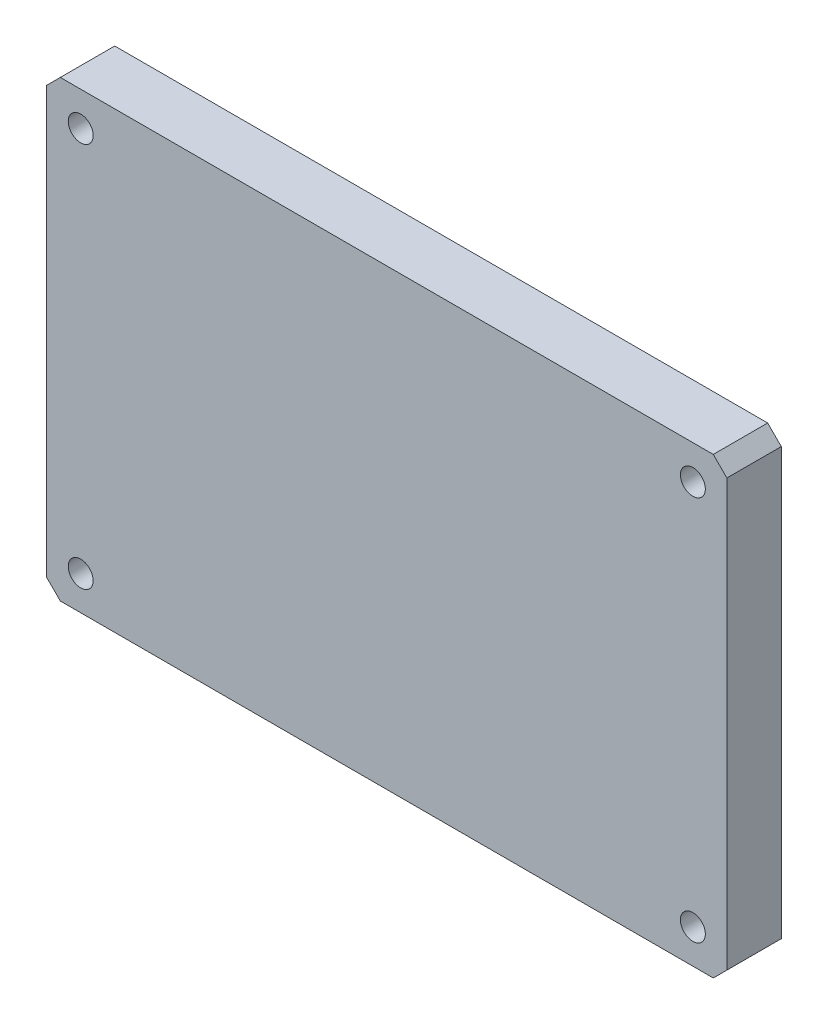
from build123d import *

# Parameters (mm, degrees)
SKETCH1_W                                         = 150
SKETCH1_H                                         = 100
BOSS_EXTRUDE1_DEPTH                               = 12
CUT_EXTRUDE3_DEPTH                                = 1
CHAMFER1_SIZE                                     = 3
HOLE_SIZE_BASED_SOCKET_HEAD_CAP_SCREW_D           = 5.5
HOLE_SIZE_BASED_SOCKET_HEAD_CAP_SCREW_CBORE_D     = 10
HOLE_SIZE_BASED_SOCKET_HEAD_CAP_SCREW_CBORE_DEPTH = 5.7


with BuildPart() as part:
    # Sketch1 → Boss-Extrude1 (new body)
    with BuildSketch(Plane.XY):
        Rectangle(SKETCH1_W, SKETCH1_H)
    extrude(amount=BOSS_EXTRUDE1_DEPTH)

    # Sketch5 → Cut-Extrude3 (cut)
    with BuildSketch(Plane(origin=(0, 0, 0), x_dir=(-1, 0, 0), z_dir=(0, 0, -1))):
        with BuildLine():
            Line((-56.0087044, -40.651312408), (-56.0087044, -24.051312408))
            ThreePointArc((-56.0087044, -24.051312408), (-56.067283044, -23.909891052), (-56.2087044, -23.851312408))
            Line((-56.2087044, -23.851312408), (-64.8087044, -23.851312408))
            ThreePointArc((-64.8087044, -23.851312408), (-64.950125756, -23.792733764), (-65.0087044, -23.651312408))
            Line((-65.0087044, -23.651312408), (-65.0087044, -17.651312408))
            ThreePointArc((-65.0087044, -17.651312408), (-64.950125756, -17.509891052), (-64.8087044, -17.451312408))
            Line((-64.8087044, -17.451312408), (-60.6087044, -17.451312408))
            ThreePointArc((-60.6087044, -17.451312408), (-60.467283044, -17.392733764), (-60.4087044, -17.251312408))
            Line((-60.4087044, -17.251312408), (-60.4087044, 4.948687592))
            ThreePointArc((-60.4087044, 4.948687592), (-60.467283044, 5.090108948), (-60.6087044, 5.148687592))
            Line((-60.6087044, 5.148687592), (-64.8087044, 5.148687592))
            ThreePointArc((-64.8087044, 5.148687592), (-64.950125756, 5.207266236), (-65.0087044, 5.348687592))
            Line((-65.0087044, 5.348687592), (-65.0087044, 11.348687592))
            ThreePointArc((-65.0087044, 11.348687592), (-64.950125756, 11.490108948), (-64.8087044, 11.548687592))
            Line((-64.8087044, 11.548687592), (-59.2087044, 11.548687592))
            ThreePointArc((-59.2087044, 11.548687592), (-59.067283044, 11.607266236), (-59.0087044, 11.748687592))
            Line((-59.0087044, 11.748687592), (-59.0087044, 36.248687592))
            ThreePointArc((-59.0087044, 36.248687592), (-58.950125756, 36.390108948), (-58.8087044, 36.448687592))
            Line((-58.8087044, 36.448687592), (-43.7087044, 36.448687592))
            ThreePointArc((-43.7087044, 36.448687592), (-43.567283044, 36.507266236), (-43.5087044, 36.648687592))
            Line((-43.5087044, 36.648687592), (-43.5087044, 39.648687592))
            ThreePointArc((-43.5087044, 39.648687592), (-43.450125756, 39.790108948), (-43.3087044, 39.848687592))
            Line((-43.3087044, 39.848687592), (-37.3087044, 39.848687592))
            ThreePointArc((-37.3087044, 39.848687592), (-37.167283044, 39.790108948), (-37.1087044, 39.648687592))
            Line((-37.1087044, 39.648687592), (-37.1087044, 36.648687592))
            ThreePointArc((-37.1087044, 36.648687592), (-37.050125756, 36.507266236), (-36.9087044, 36.448687592))
            Line((-36.9087044, 36.448687592), (-4.7087044, 36.448687592))
            ThreePointArc((-4.7087044, 36.448687592), (-4.567283044, 36.507266236), (-4.5087044, 36.648687592))
            Line((-4.5087044, 36.648687592), (-4.5087044, 39.648687592))
            ThreePointArc((-4.5087044, 39.648687592), (-4.450125756, 39.790108948), (-4.3087044, 39.848687592))
            Line((-4.3087044, 39.848687592), (1.6912956, 39.848687592))
            ThreePointArc((1.6912956, 39.848687592), (1.832716956, 39.790108948), (1.8912956, 39.648687592))
            Line((1.8912956, 39.648687592), (1.8912956, 36.648687592))
            ThreePointArc((1.8912956, 36.648687592), (1.949874244, 36.507266236), (2.0912956, 36.448687592))
            Line((2.0912956, 36.448687592), (40.2912956, 36.448687592))
            ThreePointArc((40.2912956, 36.448687592), (40.432716956, 36.507266236), (40.4912956, 36.648687592))
            Line((40.4912956, 36.648687592), (40.4912956, 39.648687592))
            ThreePointArc((40.4912956, 39.648687592), (40.549874244, 39.790108948), (40.6912956, 39.848687592))
            Line((40.6912956, 39.848687592), (46.6912956, 39.848687592))
            ThreePointArc((46.6912956, 39.848687592), (46.832716956, 39.790108948), (46.8912956, 39.648687592))
            Line((46.8912956, 39.648687592), (46.8912956, 36.648687592))
            ThreePointArc((46.8912956, 36.648687592), (46.949874244, 36.507266236), (47.0912956, 36.448687592))
            Line((47.0912956, 36.448687592), (62.1912956, 36.448687592))
            ThreePointArc((62.1912956, 36.448687592), (62.332716956, 36.390108948), (62.3912956, 36.248687592))
            Line((62.3912956, 36.248687592), (62.3912956, 11.748687592))
            ThreePointArc((62.3912956, 11.748687592), (62.449874244, 11.607266236), (62.5912956, 11.548687592))
            Line((62.5912956, 11.548687592), (68.1912956, 11.548687592))
            ThreePointArc((68.1912956, 11.548687592), (68.332716956, 11.490108948), (68.3912956, 11.348687592))
            Line((68.3912956, 11.348687592), (68.3912956, 5.348687592))
            ThreePointArc((68.3912956, 5.348687592), (68.332716956, 5.207266236), (68.1912956, 5.148687592))
            Line((68.1912956, 5.148687592), (62.5912956, 5.148687592))
            ThreePointArc((62.5912956, 5.148687592), (62.449874244, 5.090108948), (62.3912956, 4.948687592))
            Line((62.3912956, 4.948687592), (62.3912956, -17.251312408))
            ThreePointArc((62.3912956, -17.251312408), (62.449874244, -17.392733764), (62.5912956, -17.451312408))
            Line((62.5912956, -17.451312408), (68.1912956, -17.451312408))
            ThreePointArc((68.1912956, -17.451312408), (68.332716956, -17.509891052), (68.3912956, -17.651312408))
            Line((68.3912956, -17.651312408), (68.3912956, -23.651312408))
            ThreePointArc((68.3912956, -23.651312408), (68.332716956, -23.792733764), (68.1912956, -23.851312408))
            Line((68.1912956, -23.851312408), (59.5912956, -23.851312408))
            ThreePointArc((59.5912956, -23.851312408), (59.449874244, -23.909891052), (59.3912956, -24.051312408))
            Line((59.3912956, -24.051312408), (59.3912956, -40.651312408))
            ThreePointArc((59.3912956, -40.651312408), (59.332716956, -40.792733764), (59.1912956, -40.851312408))
            Line((59.1912956, -40.851312408), (-55.8087044, -40.851312408))
            ThreePointArc((-55.8087044, -40.851312408), (-55.950125756, -40.792733764), (-56.0087044, -40.651312408))
        make_face()
    extrude(amount=-CUT_EXTRUDE3_DEPTH, mode=Mode.SUBTRACT)

    # Chamfer1
    chamfer1_edges = [part.edges().sort_by_distance(p)[0] for p in [
        (75, -50, 6),
        (-75, -50, 6),
        (-75, 50, 6),
        (75, 50, 6),
    ]]
    chamfer(chamfer1_edges, length=CHAMFER1_SIZE)

    # Hole Size (%based) Socket Head Cap Screw Type1 (through all)
    with Locations(Plane(origin=(0, 0, 0), x_dir=(-1, 0, 0), z_dir=(0, 0, -1))):
        with Locations((-67.5, 42.5), (67.5, 42.5), (67.5, -42.5), (-67.5, -42.5)):
            CounterBoreHole(HOLE_SIZE_BASED_SOCKET_HEAD_CAP_SCREW_D / 2, HOLE_SIZE_BASED_SOCKET_HEAD_CAP_SCREW_CBORE_D / 2, HOLE_SIZE_BASED_SOCKET_HEAD_CAP_SCREW_CBORE_DEPTH)


solid = part.part
